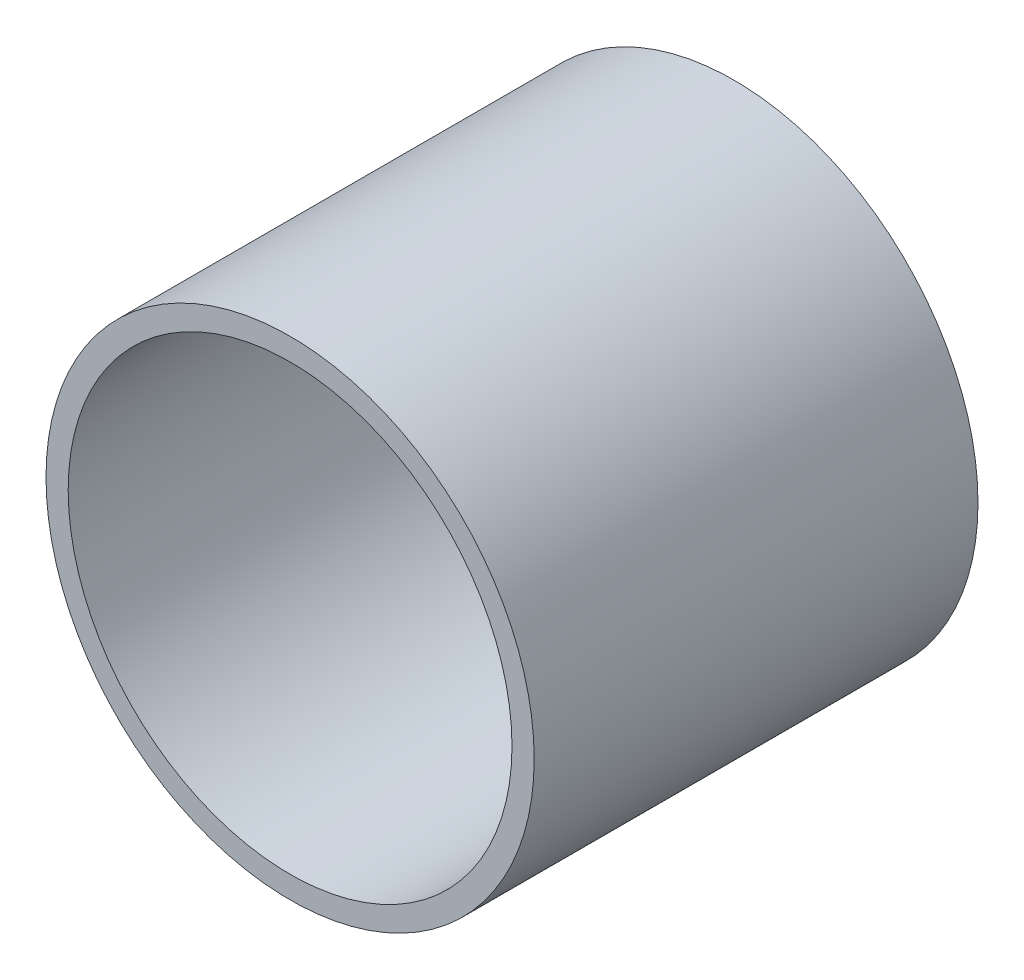
SolidWorks part; units mm, degrees
ref_plane "前视基准面" through (0, 0, 0) normal (0, 0, 1) x (1, 0, 0)
ref_plane "上视基准面" through (0, 0, 0) normal (0, 1, 0) x (1, 0, 0)
ref_plane "右视基准面" through (0, 0, 0) normal (1, 0, 0) x (0, 0, -1)
other "Configuration Table"
sketch "草图1" plane through (0, 0, 0) normal (0, 0, 1) x (1, 0, 0)
  circle A0 centre (0, 0) radius 100
  dimension "D1" = 200
extrude "拉伸-薄壁1" add sketch "草图1" along normal blind 200 thin
